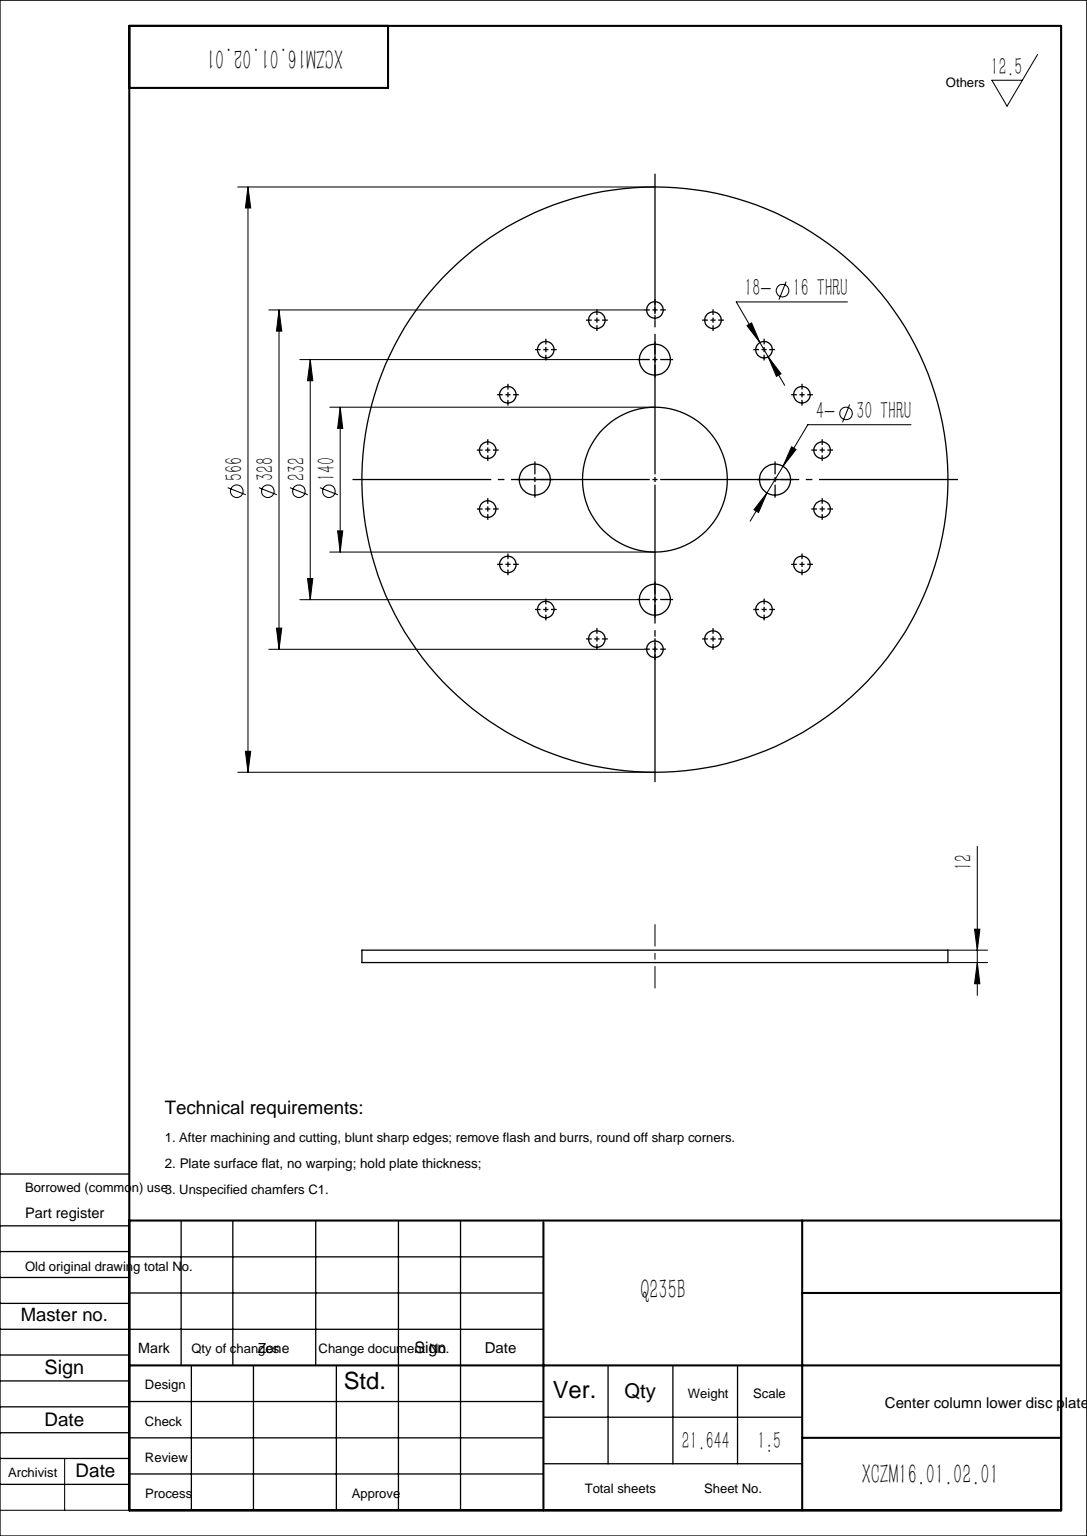
SolidWorks part; units mm, degrees
material "Q235B"
ref_plane "Front Plane" through (0, 0, 0) normal (0, 0, 1) x (1, 0, 0)
ref_plane "Top Plane" through (0, 0, 0) normal (0, 1, 0) x (1, 0, 0)
ref_plane "Right Plane" through (0, 0, 0) normal (1, 0, 0) x (0, 0, -1)
sketch "Sketch1" plane through (0, 0, 0) normal (0, 1, 0) x (1, 0, 0)
  line L0 (0, 0) -> (0, 164) construction
  line L1 (0, 0) -> (56.0913, 154.1096) construction
  line L2 (0, 0) -> (0, 116) construction
  line L3 (0, 0) -> (116, 0) construction
  circle A0 centre (0, 0) radius 70
  circle A1 centre (0, 0) radius 283
  circle A2 centre (0, 0) radius 116 construction
  circle A3 centre (0, 0) radius 164 construction
  circle A4 centre (0, 116) radius 15
  circle A5 centre (0, 164) radius 8
  circle A6 centre (56.0913, 154.1096) radius 8
  circle A7 centre (105.4172, 125.6313) radius 8
  circle A8 centre (142.0282, 82) radius 8
  circle A9 centre (161.5085, 28.4783) radius 8
  circle A10 centre (161.5085, -28.4783) radius 8
  circle A11 centre (142.0282, -82) radius 8
  circle A12 centre (105.4172, -125.6313) radius 8
  circle A13 centre (56.0913, -154.1096) radius 8
  circle A14 centre (0, -164) radius 8
  circle A15 centre (-56.0913, -154.1096) radius 8
  circle A16 centre (-105.4172, -125.6313) radius 8
  circle A17 centre (-142.0282, -82) radius 8
  circle A18 centre (-161.5085, -28.4783) radius 8
  circle A19 centre (-161.5085, 28.4783) radius 8
  circle A20 centre (-142.0282, 82) radius 8
  circle A21 centre (-105.4172, 125.6313) radius 8
  circle A22 centre (-56.0913, 154.1096) radius 8
  circle A23 centre (116, 0) radius 15
  circle A24 centre (0, -116) radius 15
  circle A25 centre (-116, 0) radius 15
  dimension "D1" = 140
  dimension "D2" = 566
  dimension "D3" = 232
  dimension "D4" = 328
  dimension "D5" = 30
  dimension "D6" = 16
  dimension "D8" = 20
  dimension "D10" = 90
  dimension "D7" = 18
  dimension "D9" = 4
extrude "Boss-Extrude1" add sketch "Sketch1" along normal blind 12
